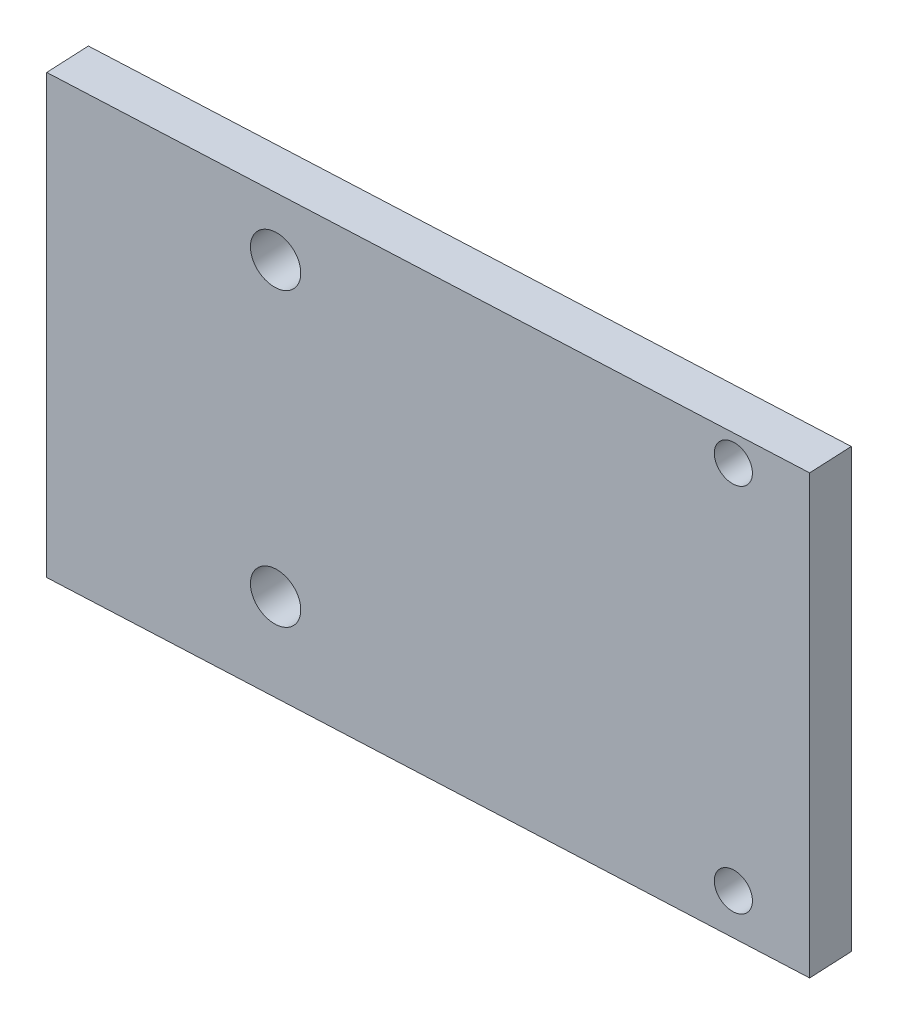
SolidWorks part; units mm, degrees
ref_plane "Front Plane" through (0, 0, 0) normal (0, 0, 1) x (1, 0, 0)
ref_plane "Top Plane" through (0, 0, 0) normal (0, 1, 0) x (1, 0, 0)
ref_plane "Right Plane" through (0, 0, 0) normal (1, 0, 0) x (0, 0, -1)
other "Configuration Table"
sketch "Sketch1" plane through (18.5233, 0, -0.4408) normal (-0.0476, 0, -0.9989) x (-0.9989, 0, 0.0476)
  line L1 (-17.4081, 324) -> (32.5919, 324)
  line L2 (-17.4081, 324) -> (-17.4081, 294)
  line L3 (-17.4081, 294) -> (32.5919, 294)
  line L4 (32.5919, 324) -> (32.5919, 294)
  line L6 (0.0919, 349) -> (35.0919, 349) construction
  line L7 (32.5919, 384) -> (32.5919, 0) construction
  dimension "D1" = 50
  dimension "D2" = 30
  dimension "D3" = 25
extrude "Boss-Extrude1" add sketch "Sketch1" against normal blind 3 contours L1 L4 L3 L2
hole_wizard "M4 Tapped Hole1" positions "Sketch2" profile "Sketch3" tap size "M4" standard "GB" end condition through all
sketch "Sketch2" plane through (0.021, 0, 0.4403) normal (-0.0476, 0, -0.9989) x (-0.9989, 0, 0.0476)
  line L0 (-0.9314, 324) -> (-0.9314, 294) construction
  line L1 (-35.9314, 324) -> (14.0686, 324) construction
  line L2 (-35.9314, 294) -> (14.0686, 294) construction
  line L4 (14.0686, 324) -> (14.0686, 294) construction
  point P0 (-0.9314, 320)
  point P2 (-0.9314, 300)
  dimension "D1" = 15
  dimension "D2" = 4
  dimension "D3" = 20
sketch "Sketch3" plane through (0.9513, 320, 0.396) normal (0, 1, 0) x (-0.9989, 0, 0.0476)
  line L0 (0, 0) -> (0, 5.3756)
  line L1 (0, 5.3756) -> (1.65, 5.3756)
  line L2 (1.65, 5.3756) -> (1.65, 0)
  line L5 (1.65, 0) -> (0, 0)
  line L11 (0, -6.35) -> (0, 107.95) construction
  dimension "通孔螺纹孔钻头直径" = 3.3
  dimension "通孔螺纹孔钻头深度" = 5.3756
cosmetic thread "Hole thread line1"
cosmetic thread "Hole thread line2"
hole_wizard "M3 Tapped Hole1" positions "Sketch4" profile "Sketch5" tap size "M3" standard "GB" end condition through all
sketch "Sketch4" plane through (0.021, 0, 0.4403) normal (-0.0476, 0, -0.9989) x (-0.9989, 0, 0.0476)
  line L0 (-35.9314, 324) -> (-35.9314, 294) construction
  line L1 (-35.9314, 294) -> (14.0686, 294) construction
  point P0 (-30.9314, 322.2)
  point P2 (-30.9314, 296.8)
  dimension "D1" = 5
  dimension "D2" = 2.8
  dimension "D3" = 25.4
  dimension "D4" = 5
sketch "Sketch5" plane through (30.9173, 322.2, -1.031) normal (0, 1, 0) x (-0.9989, 0, 0.0476)
  line L0 (0, 0) -> (0, 5.3756)
  line L1 (0, 5.3756) -> (1.25, 5.3756)
  line L2 (1.25, 5.3756) -> (1.25, 0)
  line L5 (1.25, 0) -> (0, 0)
  line L11 (0, -6.35) -> (0, 107.95) construction
  dimension "通孔螺纹孔钻头直径" = 2.5
  dimension "通孔螺纹孔钻头深度" = 5.3756
cosmetic thread "Hole thread line3"
cosmetic thread "Hole thread line4"
